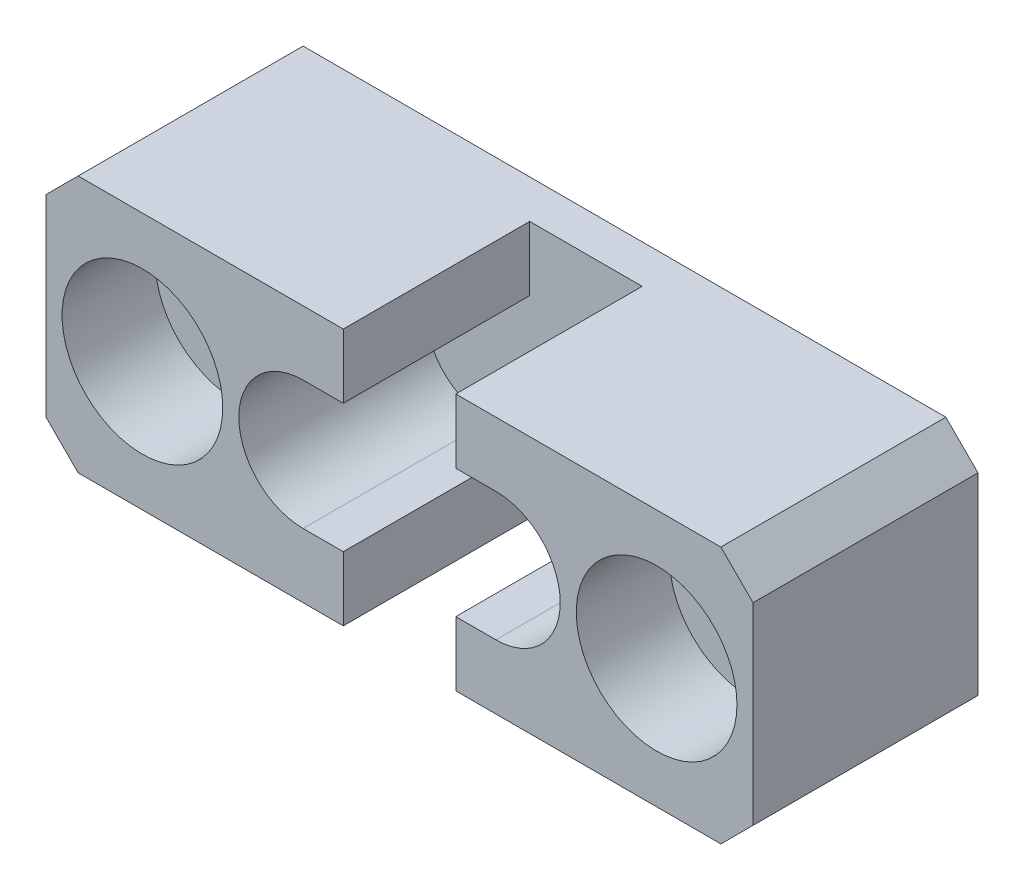
from build123d import *

# Parameters (mm, degrees)
SKETCH1_W                                            = 22
SKETCH1_H                                            = 8
BOSS_EXTRUDE1_DEPTH                                  = 7
CUT_EXTRUDE1_DEPTH                                   = 5.8
CHAMFER1_SIZE                                        = 1
HOLE_SIZE_PER_SOCKET_HEAD_CAP_SCREW_TYPE_D           = 2.9
HOLE_SIZE_PER_SOCKET_HEAD_CAP_SCREW_TYPE_CBORE_D     = 5
HOLE_SIZE_PER_SOCKET_HEAD_CAP_SCREW_TYPE_CBORE_DEPTH = 2.9


with BuildPart() as part:
    # Sketch1 → Boss-Extrude1 (new body)
    with BuildSketch(Plane.XY):
        Rectangle(SKETCH1_W, SKETCH1_H)
    extrude(amount=BOSS_EXTRUDE1_DEPTH)

    # Sketch3 → Cut-Extrude1 (cut)
    with BuildSketch(Plane.XY.offset(7)):
        with BuildLine():
            Line((-3, 2), (-1.75, 2))
            Line((-1.75, 2), (-1.75, 4))
            Line((-1.75, 4), (1.75, 4))
            Line((1.75, 4), (1.75, 2))
            Line((1.75, 2), (3, 2))
            ThreePointArc((3, 2), (5, 0), (3, -2))
            Line((3, -2), (1.75, -2))
            Line((1.75, -2), (1.75, -4))
            Line((1.75, -4), (-1.75, -4))
            Line((-1.75, -4), (-1.75, -2))
            Line((-1.75, -2), (-3, -2))
            ThreePointArc((-3, -2), (-5, 0), (-3, 2))
        make_face()
    extrude(amount=-CUT_EXTRUDE1_DEPTH, mode=Mode.SUBTRACT)

    # Chamfer1
    chamfer1_edges = [part.edges().sort_by_distance(p)[0] for p in [
        (11, -4, 3.5),
        (-11, -4, 3.5),
        (-11, 4, 3.5),
        (11, 4, 3.5),
    ]]
    chamfer(chamfer1_edges, length=CHAMFER1_SIZE)

    # Hole size per socket head cap screw type 1 (through all)
    with Locations(Plane.XY.offset(7)):
        with Locations((-8, 0), (8, 0)):
            CounterBoreHole(HOLE_SIZE_PER_SOCKET_HEAD_CAP_SCREW_TYPE_D / 2, HOLE_SIZE_PER_SOCKET_HEAD_CAP_SCREW_TYPE_CBORE_D / 2, HOLE_SIZE_PER_SOCKET_HEAD_CAP_SCREW_TYPE_CBORE_DEPTH)


solid = part.part
